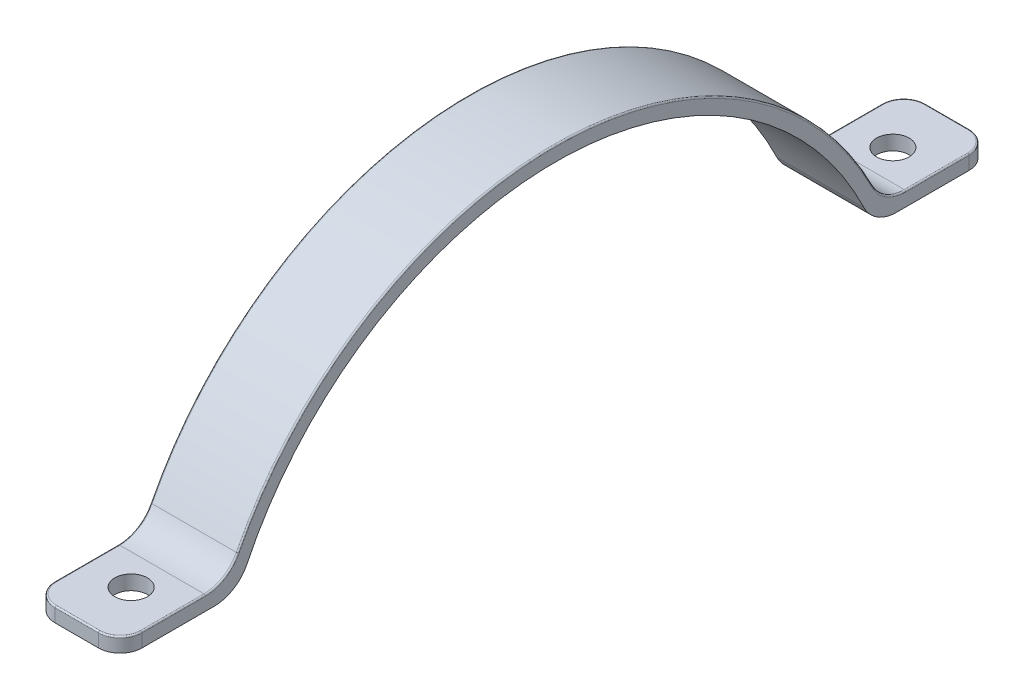
SolidWorks part; units mm, degrees
material "不锈钢304"
ref_plane "前视基准面" through (0, 0, 0) normal (0, 0, 1) x (1, 0, 0)
ref_plane "上视基准面" through (0, 0, 0) normal (0, 1, 0) x (1, 0, 0)
ref_plane "右视基准面" through (0, 0, 0) normal (1, 0, 0) x (0, 0, -1)
sketch "草图1" plane through (0, 0, 0) normal (1, 0, 0) x (0, 0, -1)
  line L0 (43.7574, 17.6592) -> (60, 17.6592)
  line L1 (45.0971, 19.6592) -> (60, 19.6592)
  line L2 (60, 19.6592) -> (60, 17.6592)
  line L3 (0, 0) -> (0, 106.9114) construction
  line L4 (-60, 19.6592) -> (-60, 17.6592)
  line L5 (-45.0971, 19.6592) -> (-60, 19.6592)
  line L6 (-43.7574, 17.6592) -> (-60, 17.6592)
  arc A0 (45.0971, 19.6592) -> (-45.0971, 19.6592) centre (0, 0) ccw
  arc A1 (43.7574, 17.6592) -> (-43.7574, 17.6592) centre (0, 0) ccw
  dimension "D1" = 120
  dimension "D2" = 2
extrude "凸台-拉伸1" add sketch "草图1" along normal mid plane 12
sketch "草图2" plane through (0, 19.6592, 0) normal (0, 1, 0) x (1, 0, 0)
  line L0 (0, 0) -> (49.4481, 0) construction
  line L1 (0, 0) -> (0, -105) construction
  circle A0 centre (0, -52.5) radius 2.25
  circle A1 centre (0, 52.5) radius 2.25
  point P7 (0, 0)
  dimension "D1" = 4.5
  dimension "D2" = 105
extrude "切除-拉伸1" cut sketch "草图2" against normal blind 12
fillet "圆角1" radius 3 4 edges at (6, 18.6592, 60) (-6, 18.6592, 60) (-6, 18.6592, -60) (6, 18.6592, -60)
fillet "圆角2" radius 5 2 edges at (0, 19.6592, -45.0971) (0, 19.6592, 45.0971)
fillet "圆角3" radius 5 2 edges at (0, 17.6592, 43.7574) (0, 17.6592, -43.7574)
fillet "圆角4" radius 0.2 16 edges at (6, 20.3945, -45.6508) (6, 19.6592, -52.6304) (5.1213, 19.6592, -59.1213) (0, 19.6592, -60) (-5.1213, 19.6592, -59.1213) (-6, 19.6592, -52.6304) (-6, 20.3945, -45.6508) (-6, 49.1958, 0) (-6, 20.3945, 45.6508) (-6, 19.6592, 52.6304) (-5.1213, 19.6592, 59.1213) (0, 19.6592, 60) (5.1213, 19.6592, 59.1213) (6, 19.6592, 52.6304) (6, 20.3945, 45.6508) (6, 49.1958, 0)
